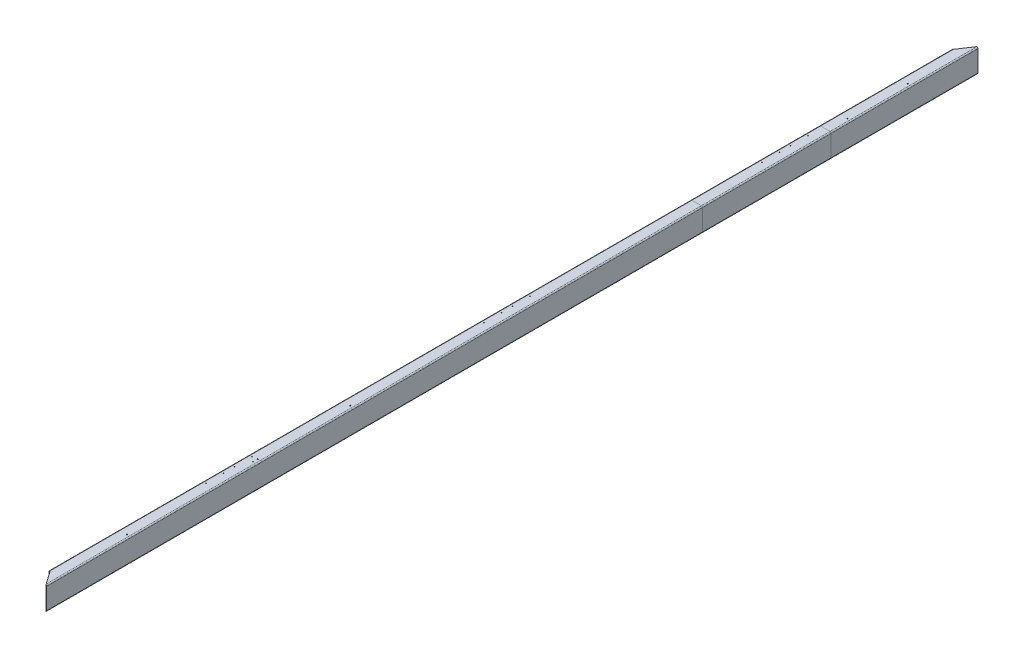
from build123d import *

# Parameters (mm, degrees)
EXTRUDE_1_DEPTH              = 1377
EXTRUDE_1_2_DEPTH            = 60
CUT_EXTRUDE_1_DEPTH          = 1441.692194745
EXTRUDE_2_DEPTH              = 1182
CUT_EXTRUDE_2_DEPTH          = 2562.075164848
HOLE_WIZARD_M3_1_AT_2_COUNT  = 2
HOLE_WIZARD_M3_1_AT_2_PITCH  = 2507.499999999
HOLE_WIZARD_M3_1_AT_3_COUNT  = 2
HOLE_WIZARD_M3_1_AT_3_PITCH  = 2582.499999999
HOLE_WIZARD_M3_1_AT_4_COUNT  = 2
HOLE_WIZARD_M3_1_AT_4_PITCH  = 2459.999999999
HOLE_WIZARD_M3_1_AT_5_COUNT  = 2
HOLE_WIZARD_M3_1_AT_5_PITCH  = 2384.999999999
HOLE_WIZARD_M3_1_AT_6_COUNT  = 2
HOLE_WIZARD_M3_1_AT_6_PITCH  = 1389.5
HOLE_WIZARD_M3_1_AT_7_COUNT  = 2
HOLE_WIZARD_M3_1_AT_7_PITCH  = 1314.5
HOLE_WIZARD_M3_1_AT_8_COUNT  = 2
HOLE_WIZARD_M3_1_AT_8_PITCH  = 1268
HOLE_WIZARD_M3_1_AT_9_COUNT  = 2
HOLE_WIZARD_M3_1_AT_9_PITCH  = 1193
HOLE_WIZARD_M3_1_AT_10_COUNT = 2
HOLE_WIZARD_M3_1_AT_10_PITCH = 122.5
HOLE_WIZARD_M3_1_AT_11_COUNT = 2
HOLE_WIZARD_M3_1_AT_11_PITCH = 197.5
HOLE_WIZARD_M3_1_AT_12_COUNT = 2
HOLE_WIZARD_M3_1_AT_12_PITCH = 75
HOLE_WIZARD_M4_2_AT_2_COUNT  = 2
HOLE_WIZARD_M4_2_AT_2_PITCH  = 397.493689191
HOLE_WIZARD_M4_2_AT_3_COUNT  = 2
HOLE_WIZARD_M4_2_AT_3_PITCH  = 418
HOLE_WIZARD_M4_2_AT_4_COUNT  = 2
HOLE_WIZARD_M4_2_AT_4_PITCH  = 958
SKETCH_14_R                  = 1.65
CUT_EXTRUDE_3_DEPTH          = 10


with BuildPart() as part:
    # 草图1 → Extrude 1 (new, symmetric)
    with BuildSketch(Plane.XY):
        with BuildLine():
            Line((-20, 50), (20, 50))
            ThreePointArc((20, 50), (23.535533906, 48.535533906), (25, 45))
            Line((25, 45), (25, -45))
            ThreePointArc((25, -45), (23.535533906, -48.535533906), (20, -50))
            Line((20, -50), (-20, -50))
            ThreePointArc((-20, -50), (-23.535533906, -48.535533906), (-25, -45))
            Line((-25, -45), (-25, 45))
            ThreePointArc((-25, 45), (-23.535533906, 48.535533906), (-20, 50))
        make_face()
        with BuildLine():
            Line((-20, 46), (20, 46))
            ThreePointArc((20, 46), (20.707106781, 45.707106781), (21, 45))
            Line((21, 45), (21, -45))
            ThreePointArc((21, -45), (20.707106781, -45.707106781), (20, -46))
            Line((20, -46), (-20, -46))
            ThreePointArc((-20, -46), (-20.707106781, -45.707106781), (-21, -45))
            Line((-21, -45), (-21, 45))
            ThreePointArc((-21, 45), (-20.707106781, 45.707106781), (-20, 46))
        make_face(mode=Mode.SUBTRACT)
    extrude(amount=EXTRUDE_1_DEPTH, both=True)


with BuildPart() as body_2:
    # 草图2 → Extrude 1 2 (new body)
    with BuildSketch(Plane.XY.offset(1377)):
        with BuildLine():
            Line((-20, -50), (20, -50))
            ThreePointArc((20, -50), (23.535533906, -48.535533906), (25, -45))
            Line((25, -45), (25, 45))
            ThreePointArc((25, 45), (23.535533906, 48.535533906), (20, 50))
            Line((20, 50), (-20, 50))
            ThreePointArc((-20, 50), (-23.535533906, 48.535533906), (-25, 45))
            Line((-25, 45), (-25, -45))
            ThreePointArc((-25, -45), (-23.535533906, -48.535533906), (-20, -50))
        make_face()
        with BuildLine():
            Line((-20, -46), (20, -46))
            ThreePointArc((20, -46), (20.707106781, -45.707106781), (21, -45))
            Line((21, -45), (21, 45))
            ThreePointArc((21, 45), (20.707106781, 45.707106781), (20, 46))
            Line((20, 46), (-20, 46))
            ThreePointArc((-20, 46), (-20.707106781, 45.707106781), (-21, 45))
            Line((-21, 45), (-21, -45))
            ThreePointArc((-21, -45), (-20.707106781, -45.707106781), (-20, -46))
        make_face(mode=Mode.SUBTRACT)
    extrude(amount=EXTRUDE_1_2_DEPTH)

    # 草图3 → 切除-拉伸1 (cut, through all)
    with BuildSketch(Plane(origin=(0, 50, 0), x_dir=(1, 0, 0), z_dir=(0, 1, 0))):
        Polygon((-20, -1377), (22.012452293, -1437), (-44.133254367, -1437), (-44.133254367, -1377), align=None)
    extrude(amount=-CUT_EXTRUDE_1_DEPTH, mode=Mode.SUBTRACT)


with BuildPart() as body_3:
    # 草图4 → 凸台-拉伸2 (new body)
    with BuildSketch(Plane(origin=(0, 0, -1377), x_dir=(-1, 0, 0), z_dir=(0, 0, -1))):
        with BuildLine():
            Line((20, -50), (-20, -50))
            ThreePointArc((-20, -50), (-23.535533906, -48.535533906), (-25, -45))
            Line((-25, -45), (-25, 45))
            ThreePointArc((-25, 45), (-23.535533906, 48.535533906), (-20, 50))
            Line((-20, 50), (20, 50))
            ThreePointArc((20, 50), (23.535533906, 48.535533906), (25, 45))
            Line((25, 45), (25, -45))
            ThreePointArc((25, -45), (23.535533906, -48.535533906), (20, -50))
        make_face()
        with BuildLine():
            Line((20, -46), (-20, -46))
            ThreePointArc((-20, -46), (-20.707106781, -45.707106781), (-21, -45))
            Line((-21, -45), (-21, 45))
            ThreePointArc((-21, 45), (-20.707106781, 45.707106781), (-20, 46))
            Line((-20, 46), (20, 46))
            ThreePointArc((20, 46), (20.707106781, 45.707106781), (21, 45))
            Line((21, 45), (21, -45))
            ThreePointArc((21, -45), (20.707106781, -45.707106781), (20, -46))
        make_face(mode=Mode.SUBTRACT)
    extrude(amount=EXTRUDE_2_DEPTH)

    # 草图5 → 切除-拉伸2 (cut, through all)
    with BuildSketch(Plane(origin=(0, 50, 0), x_dir=(1, 0, 0), z_dir=(0, 1, 0))):
        Polygon((20, 2559), (-20, 2499), (-29.87796777, 2499), (-29.87796777, 2930.227490927), (20, 2930.227490927), align=None)
    extrude(amount=-CUT_EXTRUDE_2_DEPTH, mode=Mode.SUBTRACT)

    # 草图8 → M3 螺纹孔1 (revolve, cut)
    with BuildSketch(Plane(origin=(-11, 50, -1865.499999999), x_dir=(0, 0, 1), z_dir=(1, 0, 0))):
        Polygon((0, 0), (0, 9.251075774), (1.25, 8.5), (1.25, 0.275), (1.525, 0), align=None)
    hole_wizard_m3_1 = revolve(axis=Axis((-11, 56.35, -1865.499999999), (0, -1, 0)), mode=Mode.SUBTRACT)

    # M3 螺纹孔1 at 10: M3 螺纹孔1 ×2
    with Locations(*[(0, 0, i * HOLE_WIZARD_M3_1_AT_10_PITCH) for i in range(1, HOLE_WIZARD_M3_1_AT_10_COUNT)]):
        add(hole_wizard_m3_1, mode=Mode.SUBTRACT)

    # M3 螺纹孔1 at 11: M3 螺纹孔1 ×2
    with Locations(*[(0, 0, i * HOLE_WIZARD_M3_1_AT_11_PITCH) for i in range(1, HOLE_WIZARD_M3_1_AT_11_COUNT)]):
        add(hole_wizard_m3_1, mode=Mode.SUBTRACT)

    # M3 螺纹孔1 at 12: M3 螺纹孔1 ×2
    with Locations(*[(0, 0, i * HOLE_WIZARD_M3_1_AT_12_PITCH) for i in range(1, HOLE_WIZARD_M3_1_AT_12_COUNT)]):
        add(hole_wizard_m3_1, mode=Mode.SUBTRACT)

    # 草图13 → M4 螺纹孔3 (revolve, cut)
    with BuildSketch(Plane(origin=(10, 50, -2014), x_dir=(0, 0, 1), z_dir=(1, 0, 0))):
        Polygon((0, 0), (0, 11.091420021), (1.65, 10.1), (1.65, 0.375), (2.025, 0), align=None)
    revolve(axis=Axis((10, 56.35, -2014), (0, -1, 0)), mode=Mode.SUBTRACT)

    # 草图14 → 切除-拉伸3 (cut)
    with BuildSketch(Plane(origin=(0, 50, 0), x_dir=(1, 0, 0), z_dir=(0, 1, 0))):
        with Locations(Location((10, 2272.7, 0), (0, 0, 270))):
            Circle(SKETCH_14_R)
    extrude(amount=-CUT_EXTRUDE_3_DEPTH, mode=Mode.SUBTRACT)


with BuildPart() as part_1:
    add(part.part)

    # M3 螺纹孔1 at 2: M3 螺纹孔1 ×2
    with Locations(*[(0, 0, i * HOLE_WIZARD_M3_1_AT_2_PITCH) for i in range(1, HOLE_WIZARD_M3_1_AT_2_COUNT)]):
        add(hole_wizard_m3_1, mode=Mode.SUBTRACT)

    # M3 螺纹孔1 at 3: M3 螺纹孔1 ×2
    with Locations(*[(0, 0, i * HOLE_WIZARD_M3_1_AT_3_PITCH) for i in range(1, HOLE_WIZARD_M3_1_AT_3_COUNT)]):
        add(hole_wizard_m3_1, mode=Mode.SUBTRACT)

    # M3 螺纹孔1 at 4: M3 螺纹孔1 ×2
    with Locations(*[(0, 0, i * HOLE_WIZARD_M3_1_AT_4_PITCH) for i in range(1, HOLE_WIZARD_M3_1_AT_4_COUNT)]):
        add(hole_wizard_m3_1, mode=Mode.SUBTRACT)

    # M3 螺纹孔1 at 5: M3 螺纹孔1 ×2
    with Locations(*[(0, 0, i * HOLE_WIZARD_M3_1_AT_5_PITCH) for i in range(1, HOLE_WIZARD_M3_1_AT_5_COUNT)]):
        add(hole_wizard_m3_1, mode=Mode.SUBTRACT)

    # M3 螺纹孔1 at 6: M3 螺纹孔1 ×2
    with Locations(*[(0, 0, i * HOLE_WIZARD_M3_1_AT_6_PITCH) for i in range(1, HOLE_WIZARD_M3_1_AT_6_COUNT)]):
        add(hole_wizard_m3_1, mode=Mode.SUBTRACT)

    # M3 螺纹孔1 at 7: M3 螺纹孔1 ×2
    with Locations(*[(0, 0, i * HOLE_WIZARD_M3_1_AT_7_PITCH) for i in range(1, HOLE_WIZARD_M3_1_AT_7_COUNT)]):
        add(hole_wizard_m3_1, mode=Mode.SUBTRACT)

    # M3 螺纹孔1 at 8: M3 螺纹孔1 ×2
    with Locations(*[(0, 0, i * HOLE_WIZARD_M3_1_AT_8_PITCH) for i in range(1, HOLE_WIZARD_M3_1_AT_8_COUNT)]):
        add(hole_wizard_m3_1, mode=Mode.SUBTRACT)

    # M3 螺纹孔1 at 9: M3 螺纹孔1 ×2
    with Locations(*[(0, 0, i * HOLE_WIZARD_M3_1_AT_9_PITCH) for i in range(1, HOLE_WIZARD_M3_1_AT_9_COUNT)]):
        add(hole_wizard_m3_1, mode=Mode.SUBTRACT)

    # 草图11 → M4 螺纹孔2 (revolve, cut)
    with BuildSketch(Plane(origin=(10, 50, 119), x_dir=(0, 0, 1), z_dir=(1, 0, 0))):
        Polygon((0, 0), (0, 11.091420021), (1.65, 10.1), (1.65, 0.375), (2.025, 0), align=None)
    hole_wizard_m4_2 = revolve(axis=Axis((10, 56.35, 119), (0, -1, 0)), mode=Mode.SUBTRACT)

    # M4 螺纹孔2 at 2: M4 螺纹孔2 ×2
    with Locations(*[(0, 0, i * HOLE_WIZARD_M4_2_AT_2_PITCH) for i in range(1, HOLE_WIZARD_M4_2_AT_2_COUNT)]):
        add(hole_wizard_m4_2, mode=Mode.SUBTRACT)

    # M4 螺纹孔2 at 3: M4 螺纹孔2 ×2
    with Locations(*[(0, 0, i * HOLE_WIZARD_M4_2_AT_3_PITCH) for i in range(1, HOLE_WIZARD_M4_2_AT_3_COUNT)]):
        add(hole_wizard_m4_2, mode=Mode.SUBTRACT)

    # M4 螺纹孔2 at 4: M4 螺纹孔2 ×2
    with Locations(*[(0, 0, i * HOLE_WIZARD_M4_2_AT_4_PITCH) for i in range(1, HOLE_WIZARD_M4_2_AT_4_COUNT)]):
        add(hole_wizard_m4_2, mode=Mode.SUBTRACT)


with BuildPart() as body_2_1:
    add(body_2.part)

    # Combine 1: union part
    add(part_1.part)


solid = Compound([body_3.part, body_2_1.part])
